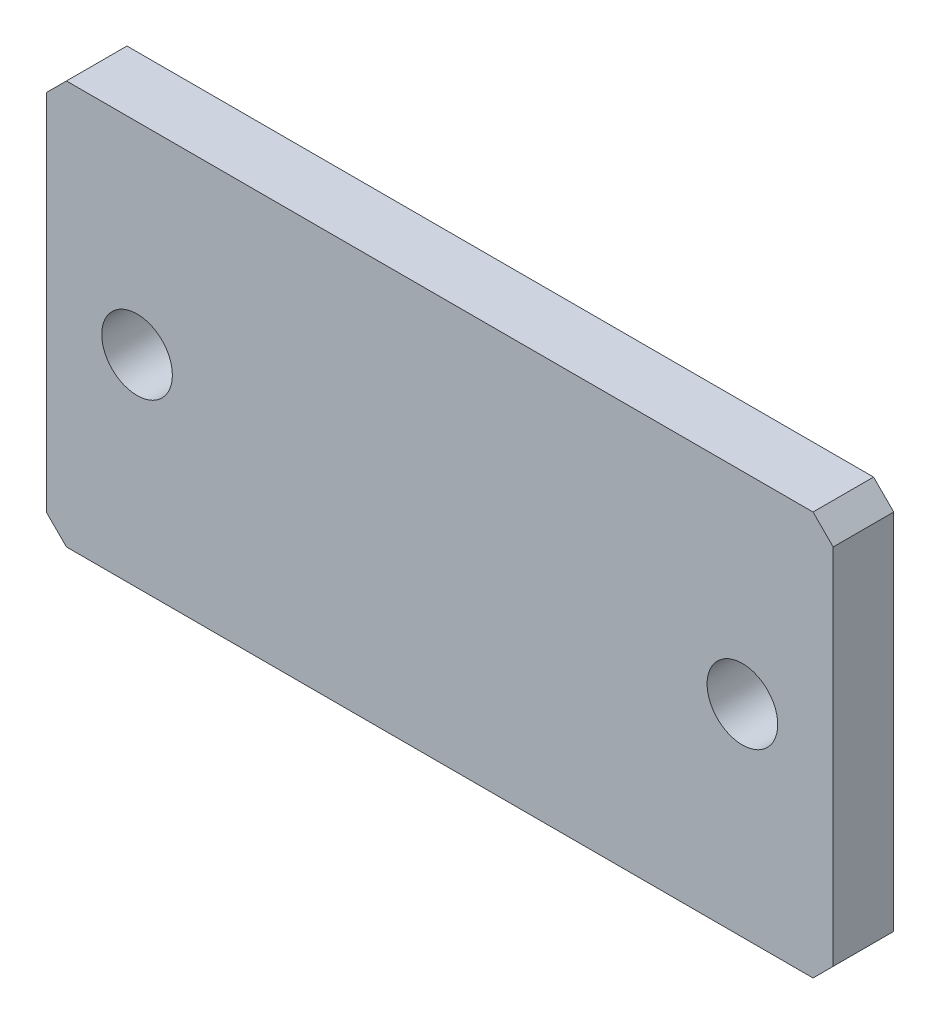
SolidWorks part; units mm, degrees
material "304"
ref_plane "Front Plane" through (0, 0, 0) normal (0, 0, 1) x (1, 0, 0)
ref_plane "Top Plane" through (0, 0, 0) normal (0, 1, 0) x (1, 0, 0)
ref_plane "Right Plane" through (0, 0, 0) normal (1, 0, 0) x (0, 0, -1)
sketch "Sketch1" plane through (0, 0, 0) normal (0, 0, 1) x (1, 0, 0)
  line L0 (-19.5, 0) -> (19.5, 0) construction
  line L1 (-19.5, -10) -> (19.5, -10)
  line L2 (-19.5, -10) -> (-19.5, 10)
  line L3 (-19.5, 10) -> (19.5, 10)
  line L4 (19.5, -10) -> (19.5, 10)
  line L5 (-19.5, -10) -> (19.5, 10) construction
  line L6 (-19.5, 10) -> (19.5, -10) construction
  circle A0 centre (-15, 0) radius 1.75
  circle A1 centre (15, 0) radius 1.75
  point P0 (0, 0)
  dimension "D3" = 3.5
  dimension "D4" = 3.5
  dimension "D5" = 30
  dimension "D6" = 15
  dimension "D1" = 39
  dimension "D2" = 20
extrude "Boss-Extrude1" add sketch "Sketch1" along normal blind 3
chamfer "Chamfer1" distance 1 angle 45 4 edges at (19.5, -10, 1.5) (19.5, 10, 1.5) (-19.5, -10, 1.5) (-19.5, 10, 1.5)
